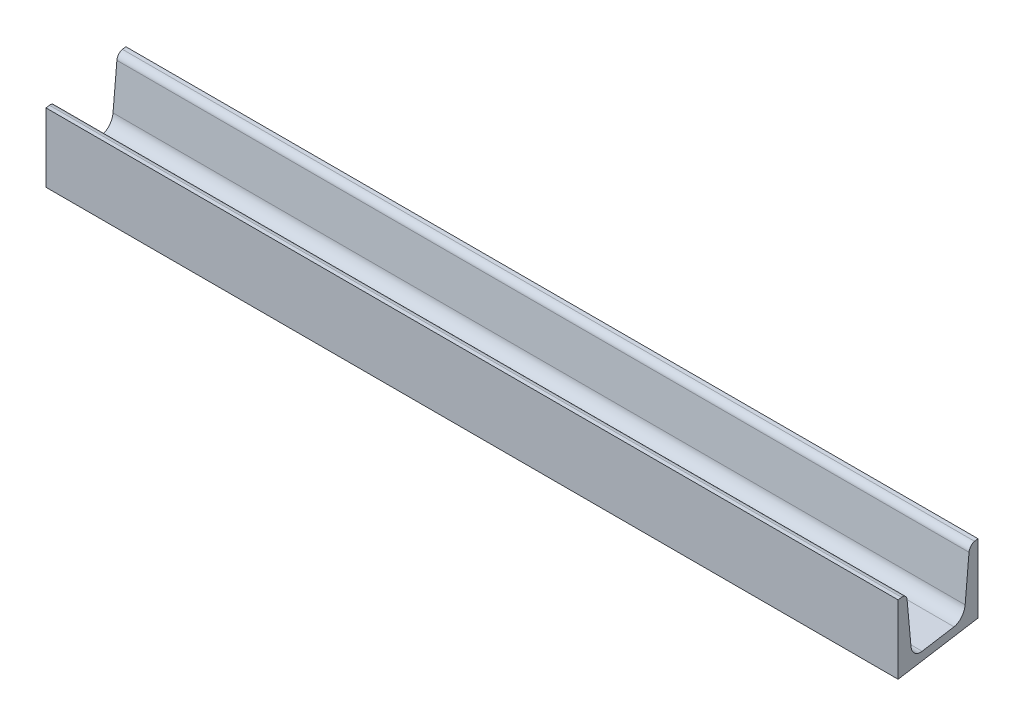
from build123d import *

# Parameters (mm, degrees)
GB_T_707_1988_HOT_ROLLED_CHANNEL_05_1_DEPTH = 1000
CUT_EXTRUDE6_DEPTH                          = 504.854145562
CUT_EXTRUDE6_DEPTH_BACK                     = 504.854145562


with BuildPart() as part:
    # Sketch1 → GB/T 707-1988 hot-rolled channel 05(1) (new body)
    with BuildSketch(Plane.YZ.offset(-500)):
        with BuildLine():
            Line((37, 50), (0, 50))
            Line((0, 50), (0, 0))
            Line((0, 0), (37, 0))
            Line((37, 0), (37, 2.140642022))
            ThreePointArc((37, 2.140642022), (36.101006889, 4.482599144), (33.865849621, 5.621468656))
            Line((33.865849621, 5.621468656), (10.768300757, 8.049118866))
            ThreePointArc((10.768300757, 8.049118866), (6.297986222, 10.326857889), (4.5, 15.010772133))
            Line((4.5, 15.010772133), (4.5, 34.989227867))
            ThreePointArc((4.5, 34.989227867), (6.297986222, 39.673142111), (10.768300757, 41.950881134))
            Line((10.768300757, 41.950881134), (33.865849621, 44.378531344))
            ThreePointArc((33.865849621, 44.378531344), (36.101006889, 45.517400856), (37, 47.859357978))
            Line((37, 47.859357978), (37, 50))
        make_face()
    extrude(amount=GB_T_707_1988_HOT_ROLLED_CHANNEL_05_1_DEPTH)

    # Sketch4 → Cut-Extrude6 (cut, two sides: drawn at the far end of the back side and taken through both)
    with BuildSketch(Plane.XZ.offset(-CUT_EXTRUDE6_DEPTH_BACK)):
        Polygon((-500, 50), (-500, 0), (-492.972958265, 50), align=None)
        Polygon((500, 50), (-34.511240341, 50), (-41.538282077, 0), (500, 0), align=None)
    extrude(amount=CUT_EXTRUDE6_DEPTH + CUT_EXTRUDE6_DEPTH_BACK, mode=Mode.SUBTRACT)


solid = part.part
